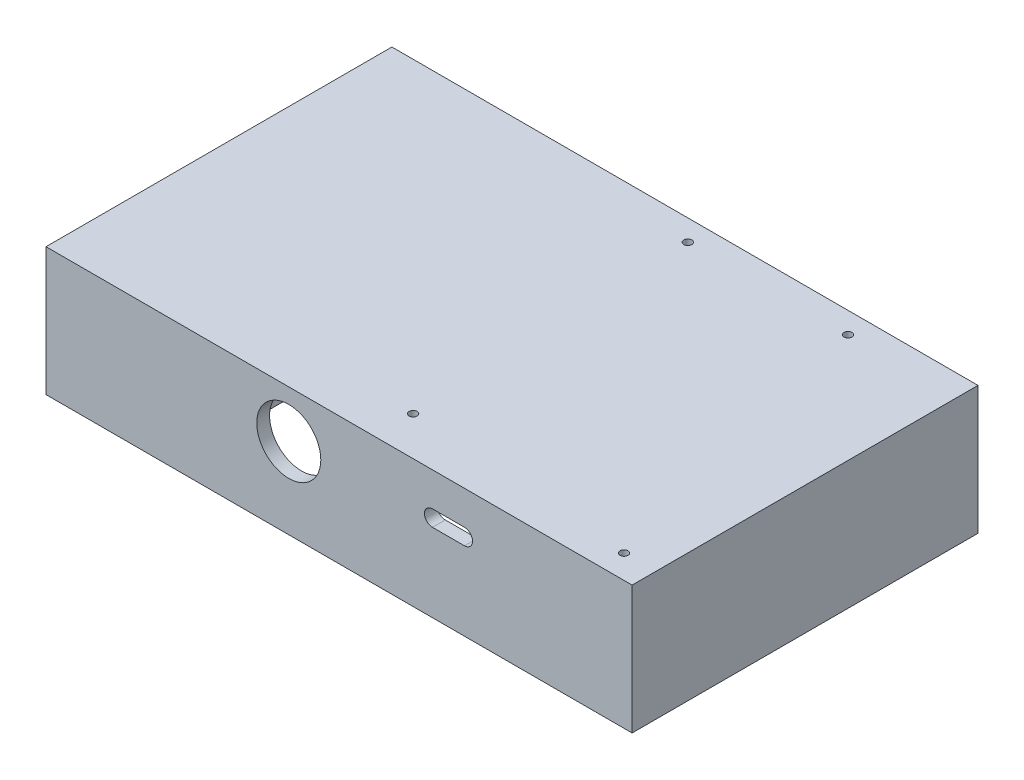
SolidWorks part; units mm, degrees
ref_plane "Front Plane" through (0, 0, 0) normal (0, 0, 1) x (1, 0, 0)
ref_plane "Top Plane" through (0, 0, 0) normal (0, 1, 0) x (1, 0, 0)
ref_plane "Right Plane" through (0, 0, 0) normal (1, 0, 0) x (0, 0, -1)
other "Configuration Table"
sketch "Sketch2" plane through (0, 0, 0) normal (0, 1, 0) x (1, 0, 0)
  line L0 (-183, -108) -> (183, -108)
  line L1 (-175, 100) -> (175, 100)
  line L2 (-175, 100) -> (-175, -100)
  line L3 (-175, -100) -> (175, -100)
  line L4 (175, 100) -> (175, -100)
  line L5 (0, -100) -> (0, 100) construction
  line L6 (-175, 0) -> (175, 0) construction
  line L7 (183, 108) -> (183, -108)
  line L8 (-183, 108) -> (183, 108)
  line L9 (-183, 108) -> (-183, -108)
  point P0 (0, 0)
  dimension "D1" = 200
  dimension "D2" = 350
  dimension "D3" = 8
extrude "Boss-Extrude1" add sketch "Sketch2" along normal blind 80
sketch "Sketch3" plane through (0, 80, 0) normal (0, 1, 0) x (1, 0, 0)
  line L4 (-183, 108) -> (-183, -108)
  line L5 (-183, -108) -> (183, -108)
  line L6 (183, -108) -> (183, 108)
  line L7 (183, 108) -> (-183, 108)
  line L8 (-183, 108) -> (-183, -108)
  line L9 (-183, -108) -> (183, -108)
  line L10 (183, -108) -> (183, 108)
  line L11 (183, 108) -> (-183, 108)
  dimension "D1" = 0
sketch "Sketch4" plane through (0, 80, 0) normal (0, 1, 0) x (1, 0, 0)
  line L4 (-183, 108) -> (-183, -108)
  line L5 (-183, -108) -> (183, -108)
  line L6 (183, -108) -> (183, 108)
  line L7 (183, 108) -> (-183, 108)
  line L8 (-183, 108) -> (-183, -108)
  line L9 (-183, -108) -> (183, -108)
  line L10 (183, -108) -> (183, 108)
  line L11 (183, 108) -> (-183, 108)
  line L12 (-183, 108) -> (-183, -108)
  line L13 (-183, -108) -> (183, -108)
  line L14 (183, -108) -> (183, 108)
  line L15 (183, 108) -> (-183, 108)
  line L16 (-183, 108) -> (-183, -108)
  line L17 (-183, -108) -> (183, -108)
  line L18 (183, -108) -> (183, 108)
  line L19 (183, 108) -> (-183, 108)
  line M13 (-175, 100) -> (175, 100)
  line M14 (175, 100) -> (175, -100)
  line M15 (175, -100) -> (-175, -100)
  line M16 (-175, -100) -> (-175, 100)
  dimension "D1" = 0
  dimension "D2" = 0
extrude "Boss-Extrude2" add sketch "Sketch4" against normal blind 2 contours M13 M16 M15 M14
sketch "Sketch5" plane through (0, 0, 108) normal (0, 0, 1) x (1, 0, 0)
  line L0 (58.3395, 53.9011) -> (78.3395, 53.9011) construction
  line L1 (58.3395, 58.9011) -> (78.3395, 58.9011)
  line L2 (58.3395, 48.9011) -> (78.3395, 48.9011)
  arc A0 (58.3395, 58.9011) -> (58.3395, 48.9011) centre (58.3395, 53.9011) ccw
  arc A1 (78.3395, 48.9011) -> (78.3395, 58.9011) centre (78.3395, 53.9011) ccw
  point P2 (68.3395, 53.9011)
  dimension "D2" = 5
  dimension "D1" = 20
extrude "Cut-Extrude1" cut sketch "Sketch5" against normal mid plane 122
sketch "Sketch6" plane through (0, 0, -100) normal (0, 0, 1) x (1, 0, 0)
  line L1 (-60.152, 67.0657) -> (59.848, 67.0657)
  line L2 (-60.152, 67.0657) -> (-60.152, 17.0657)
  line L3 (-60.152, 17.0657) -> (59.848, 17.0657)
  line L4 (59.848, 67.0657) -> (59.848, 17.0657)
  line L5 (-0.152, 17.0657) -> (-0.152, 67.0657) construction
  line L6 (-60.152, 42.0657) -> (59.848, 42.0657) construction
  point P0 (-0.152, 42.0657)
  dimension "D1" = 50
  dimension "D2" = 120
extrude "Cut-Extrude2" cut sketch "Sketch6" against normal mid plane 122
sketch "Sketch7" plane through (0, 78, 0) normal (0, -1, 0) x (1, 0, 0)
  line L1 (175, -100) -> (175, 100) construction
  line L2 (-175, -100) -> (175, -100) construction
  circle A1 centre (115, -94.8) radius 2.5
  circle A2 centre (115, -94.8) radius 5
  circle A3 centre (15, -94.8) radius 5
  circle A4 centre (15, -94.8) radius 2.5
  dimension "D1" = 5
  dimension "D2" = 10
  dimension "D3" = 60
  dimension "D4" = 5.2
  dimension "D5" = 2
extrude "Boss-Extrude6" add sketch "Sketch7" along normal blind 11
sketch "Sketch8" plane through (0, 67, 0) normal (0, -1, 0) x (1, 0, 0)
  circle A0 centre (15, -94.8) radius 2.5
  circle A1 centre (115, -94.8) radius 2.5
  dimension "D1" = 5
extrude "Cut-Extrude3" cut sketch "Sketch8" against normal through all
sketch "Sketch9" plane through (0, 78, 0) normal (0, -1, 0) x (1, 0, 0)
  circle A0 centre (21.9655, 83.7052) radius 5
  dimension "D1" = 10
sketch "Sketch10" plane through (0, 78, 0) normal (0, -1, 0) x (1, 0, 0)
  circle A0 centre (163.1624, 93.1995) radius 5
  dimension "D1" = 10
extrude "Boss-Extrude7" add sketch "Sketch10" along normal blind 11
extrude "Boss-Extrude8" add sketch "Sketch9" along normal blind 11
sketch "Sketch11" plane through (0, 67, 0) normal (0, -1, 0) x (1, 0, 0)
  circle A0 centre (21.9655, 83.7052) radius 2.5
  circle A1 centre (163.1624, 93.1995) radius 2.5
  dimension "D1" = 5
  dimension "D2" = 5
extrude "Cut-Extrude4" cut sketch "Sketch11" against normal through all
sketch "Sketch12" plane through (0, 78, 0) normal (0, -1, 0) x (1, 0, 0)
  line L0 (-94.0911, 100) -> (-94.0911, -100)
  line L1 (175, 100) -> (-175, 100) construction
  line L2 (-175, -100) -> (175, -100) construction
extrude "Extrude-Thin1" add sketch "Sketch12" along normal blind 66 thin thin type mid plane wall 2
sketch "Sketch13" plane through (0, 0, 0) normal (0, 0, 1) x (1, 0, 0)
  line L0 (-95.0911, 78) -> (-175, 78) construction
  line L1 (-174.346, 33) -> (-94.436, 33)
  line L2 (-174.346, 33) -> (-174.346, 78)
  line L3 (-174.346, 78) -> (-94.436, 78)
  line L4 (-94.436, 33) -> (-94.436, 78)
  line L5 (-134.391, 78) -> (-134.391, 33) construction
  line L6 (-174.346, 55.5) -> (-94.436, 55.5) construction
  point P280 (-134.391, 55.5)
  dimension "D1" = 79.91
  dimension "D2" = 45
ref_plane "Plane1" through (0, 0, 40) normal (0, 0, 1) x (1, 0, 0)
sketch "Sketch14" plane through (0, 0, 40) normal (0, 0, 1) x (1, 0, 0)
  line L4 (-174.346, 33) -> (-94.436, 33)
  line L5 (-94.436, 33) -> (-94.436, 78)
  line L6 (-94.436, 78) -> (-174.346, 78)
  line L7 (-174.346, 78) -> (-174.346, 33)
  line L8 (-174.346, 33) -> (-94.436, 33)
  line L9 (-94.436, 33) -> (-94.436, 78)
  line L10 (-94.436, 78) -> (-174.346, 78)
  line L11 (-174.346, 78) -> (-174.346, 33)
  dimension "D1" = 0
extrude "Boss-Extrude9" add sketch "Sketch14" along normal mid plane 4
pattern_linear "LPattern1" count 3 spacing 50 along (0, 0, -1) of "Boss-Extrude9"
sketch "Sketch15" plane through (0, 0, 38) normal (0, 0, -1) x (-1, 0, 0)
  circle A1 centre (134.391, 39.0715) radius 33.4721
extrude "Cut-Extrude5" cut sketch "Sketch15" along normal blind 114 and the other way blind 26
sketch "Sketch16" plane through (0, 0, 108) normal (0, 0, 1) x (1, 0, 0)
  circle A0 centre (-31.3935, 50.4907) radius 20
  dimension "D1" = 40
extrude "Cut-Extrude6" cut sketch "Sketch16" against normal blind 114
sketch "Sketch18" plane through (0, 78, 0) normal (0, -1, 0) x (1, 0, 0)
  line L1 (-67.8587, 50.3925) -> (4.3666, 50.3925)
  line L2 (-67.8587, 50.3925) -> (-67.8587, 34.3424)
  line L3 (-67.8587, 34.3424) -> (4.3666, 34.3424)
  line L4 (4.3666, 50.3925) -> (4.3666, 34.3424)
  line L5 (-31.7461, 34.3424) -> (-31.7461, 50.3925) construction
  line L6 (-67.8587, 42.3674) -> (4.3666, 42.3674) construction
  point P460 (-31.7461, 42.3674)
sketch "Sketch20" plane through (0, 78, 0) normal (0, -1, 0) x (1, 0, 0)
  line L1 (64.084, -43.1157) -> (-49.7431, -43.1157)
  line L2 (64.084, -43.1157) -> (64.084, -70.782)
  line L3 (64.084, -70.782) -> (-49.7431, -70.782)
  line L4 (-49.7431, -43.1157) -> (-49.7431, -70.782)
  line L5 (7.1705, -70.782) -> (7.1705, -43.1157) construction
  line L6 (64.084, -56.9489) -> (-49.7431, -56.9489) construction
  point P276 (7.1705, -56.9489)
extrude "Boss-Extrude12" add sketch "Sketch20" along normal blind 41
sketch "Sketch21" plane through (0, 0, -70.782) normal (0, 0, -1) x (-1, 0, 0)
  circle A0 centre (-47.3991, 53.3018) radius 4.7206
  circle A1 centre (-23.2903, 53.3018) radius 4.7206
  circle A2 centre (5.2453, 53.3018) radius 4.7206
  circle A3 centre (26.8297, 53.3018) radius 4.7206
extrude "Boss-Extrude13" add sketch "Sketch21" along normal blind 10
